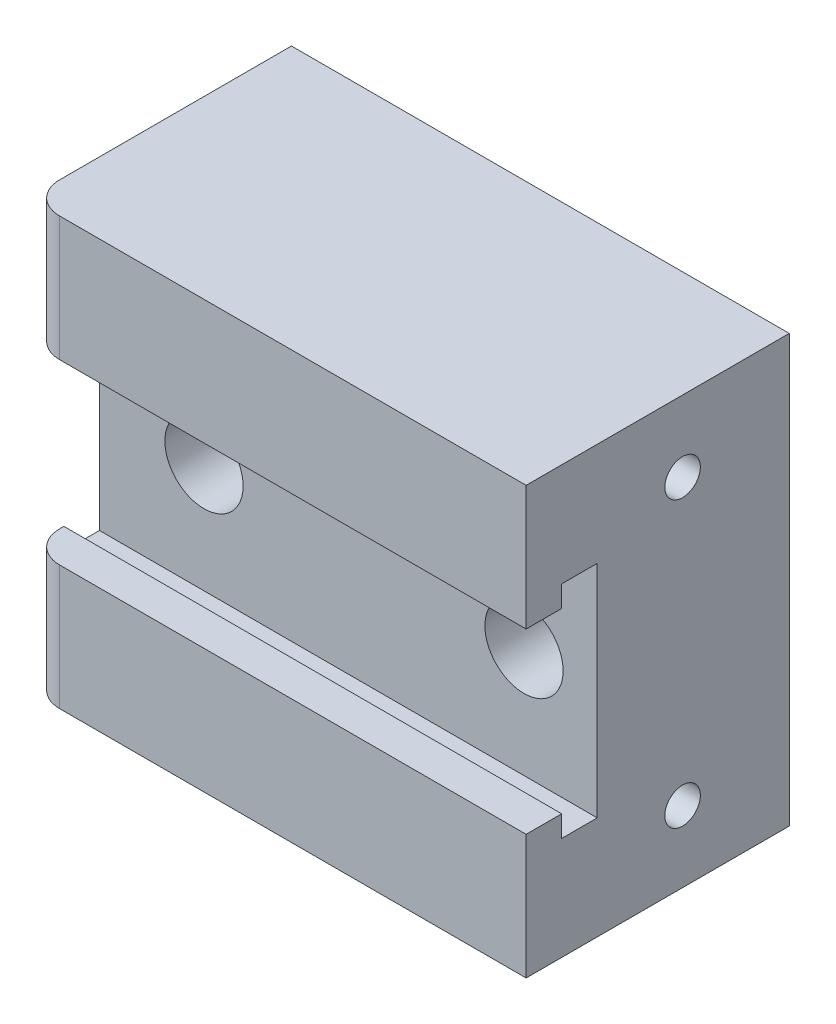
from build123d import *

# Parameters (mm, degrees)
SKETCH1_W                                           = 70
SKETCH1_H                                           = 60
BOSS_EXTRUDE1_DEPTH                                 = 37
CUT_EXTRUDE2_DEPTH                                  = 89.196341816
M6_TAPPED_HOLE1_D                                   = 5
M6_TAPPED_HOLE1_DEPTH                               = 15
M6_TAPPED_HOLE1_TIP                                 = 1.502151548
FILLET1_R                                           = 4.4
CBORE_FOR_M6_HEX_SOCKET_HEAD_CAP_SCREW1_D           = 6.6
CBORE_FOR_M6_HEX_SOCKET_HEAD_CAP_SCREW1_CBORE_D     = 11
CBORE_FOR_M6_HEX_SOCKET_HEAD_CAP_SCREW1_CBORE_DEPTH = 25


with BuildPart() as part:
    # Sketch1 → Boss-Extrude1 (new body)
    with BuildSketch(Plane.XY):
        with Locations((-25.437479048, -8.853503185)):
            Rectangle(SKETCH1_W, SKETCH1_H)
    extrude(amount=BOSS_EXTRUDE1_DEPTH)

    # Sketch3 → Cut-Extrude2 (cut, through all)
    with BuildSketch(Plane(origin=(9.562520952, 0, 0), x_dir=(0, 0, -1), z_dir=(1, 0, 0))):
        Polygon((-32, -24.353503185), (-27, -24.353503185), (-27, 6.646496815), (-32, 6.646496815), (-32, 3.646496815), (-37, 3.646496815), (-37, -21.353503185), (-32, -21.353503185), align=None)
    extrude(amount=-CUT_EXTRUDE2_DEPTH, mode=Mode.SUBTRACT)

    # M6 Tapped Hole1
    with Locations(Plane(origin=(9.562520952, 0, 0), x_dir=(0, 0, -1), z_dir=(1, 0, 0))):
        with Locations((-15, -28.853503185), (-15, 11.146496815)):
            Hole(M6_TAPPED_HOLE1_D / 2, depth=M6_TAPPED_HOLE1_DEPTH)
            with Locations((0, 0, -(M6_TAPPED_HOLE1_DEPTH + M6_TAPPED_HOLE1_TIP / 2))):  # 118° drill point
                Cone(0, M6_TAPPED_HOLE1_D / 2, M6_TAPPED_HOLE1_TIP, mode=Mode.SUBTRACT)

    # Fillet1
    fillet1_edges = [part.edges().sort_by_distance(p)[0] for p in [
        (-60.437479048, -30.103503185, 37),
        (-60.437479048, 12.396496815, 37),
    ]]
    fillet(fillet1_edges, radius=FILLET1_R)

    # CBORE for M6 Hex Socket Head Cap Screw1 (through all)
    with Locations(Plane.XY.offset(37)):
        with Locations((-0.737479048, -8.853503185), (-45.737479048, -8.853503185)):
            CounterBoreHole(CBORE_FOR_M6_HEX_SOCKET_HEAD_CAP_SCREW1_D / 2, CBORE_FOR_M6_HEX_SOCKET_HEAD_CAP_SCREW1_CBORE_D / 2, CBORE_FOR_M6_HEX_SOCKET_HEAD_CAP_SCREW1_CBORE_DEPTH)


solid = part.part
